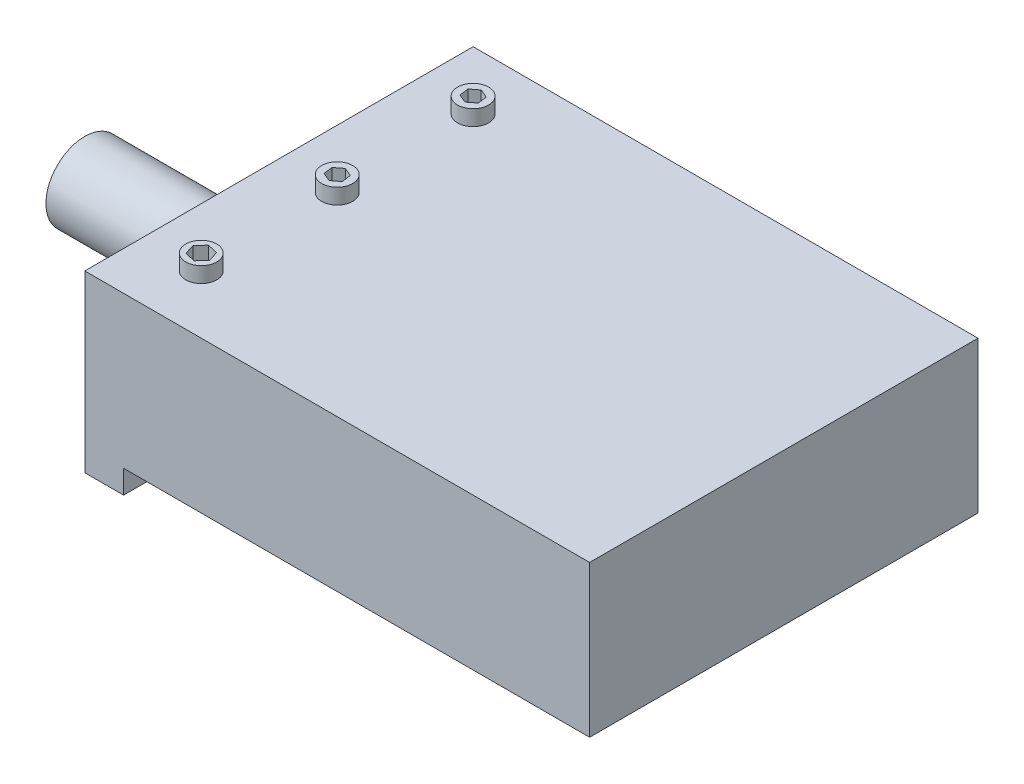
from build123d import *

# Parameters (mm, degrees)
SKETCH1_W           = 70
SKETCH1_H           = 100
BOSS_EXTRUDE1_DEPTH = 30
SKETCH2_R           = 4
BOSS_EXTRUDE2_DEPTH = 4
SKETCH3_R           = 10
BOSS_EXTRUDE3_DEPTH = 50
SKETCH4_W           = 70
SKETCH4_H           = 100
BOSS_EXTRUDE4_DEPTH = 15
SKETCH5_W           = 134.250739562
SKETCH5_H           = 64.864054132
CUT_EXTRUDE1_DEPTH  = 130
CUT_EXTRUDE2_REACH  = 189.566
SKETCH6_W           = 60
SKETCH6_H           = 6
SKETCH7_W           = 100
SKETCH7_H           = 39
BOSS_EXTRUDE5_DEPTH = 60


with BuildPart() as part:
    # Sketch1 → Boss-Extrude1 (new body)
    with BuildSketch(Plane(origin=(0, 0, 0), x_dir=(1, 0, 0), z_dir=(0, 1, 0))):
        Rectangle(SKETCH1_W, SKETCH1_H)
    extrude(amount=BOSS_EXTRUDE1_DEPTH)

    # Sketch2 → Boss-Extrude2 (add)
    # profile 1 of 3: a face of its own
    with BuildSketch(Plane(origin=(0, 30, 0), x_dir=(1, 0, 0), z_dir=(0, 1, 0))):
        with Locations(Location((20, -35, 0), (0, 0, 270))):
            Circle(SKETCH2_R)
        Polygon((21.913058762, -37.035169602), (22.719037957, -34.360827314), (20.805979195, -32.325657712), (18.086941238, -32.964830398), (17.280962043, -35.639172686), (19.194020805, -37.674342288), align=None, mode=Mode.SUBTRACT)
    # profile 2 of 3: a face of its own
    with BuildSketch(Plane(origin=(0, 30, 0), x_dir=(1, 0, 0), z_dir=(0, 1, 0))):
        with Locations(Location((20, 0, 0), (0, 0, 270))):
            Circle(SKETCH2_R)
        Polygon((21.913058762, -1.47020522), (22.229764451, 0.921654877), (20.316705689, 2.391860097), (18.086941238, 1.47020522), (17.770235549, -0.921654877), (19.683294311, -2.391860097), align=None, mode=Mode.SUBTRACT)
    # profile 3 of 3: a face of its own
    with BuildSketch(Plane(origin=(0, 30, 0), x_dir=(1, 0, 0), z_dir=(0, 1, 0))):
        with Locations(Location((20, 35, 0), (0, 0, 270))):
            Circle(SKETCH2_R)
        Polygon((21.913058762, 33.534680981), (22.225532876, 35.924097978), (20.312474114, 37.389416996), (18.086941238, 36.465319019), (17.774467124, 34.075902022), (19.687525886, 32.610583004), align=None, mode=Mode.SUBTRACT)
    extrude(amount=BOSS_EXTRUDE2_DEPTH)

    # Sketch3 → Boss-Extrude3 (add)
    with BuildSketch(Plane(origin=(35, 0, 0), x_dir=(0, 0, -1), z_dir=(1, 0, 0))):
        Circle(SKETCH3_R)
    extrude(amount=BOSS_EXTRUDE3_DEPTH)

    # Sketch4 → Boss-Extrude4 (add)
    with BuildSketch(Plane.XZ):
        Rectangle(SKETCH4_W, SKETCH4_H)
    extrude(amount=BOSS_EXTRUDE4_DEPTH)

    # Mirror1: part across plane


with BuildPart() as part_1:
    add(part.part)
    add(part.part.mirror(Plane(origin=(-35, 30, -50), x_dir=(0, 0, 1), z_dir=(1, 0, 0))))

    # Sketch5 → Cut-Extrude1 (cut)
    with BuildSketch(Plane.ZY.offset(35)):
        with Locations((0.773607985, 10.636315649)):
            Rectangle(SKETCH5_W, SKETCH5_H)
    extrude(amount=-CUT_EXTRUDE1_DEPTH, mode=Mode.SUBTRACT)

    # Sketch6 → Cut-Extrude2 (cut, up to next)
    with BuildSketch(Plane.XY.offset(50), mode=Mode.PRIVATE) as cut_extrude2_sk1:
        with Locations((-65, -12)):
            Rectangle(SKETCH6_W, SKETCH6_H)
    cut_extrude2_tool1 = extrude(cut_extrude2_sk1.sketch, amount=-CUT_EXTRUDE2_REACH, mode=Mode.PRIVATE) & part_1.part
    add(cut_extrude2_tool1.solids().sort_by_distance((-65, -12, 50))[0], mode=Mode.SUBTRACT)

    # Sketch7 → Boss-Extrude5 (add)
    with BuildSketch(Plane(origin=(-35, 0, 0), x_dir=(0, 0, -1), z_dir=(1, 0, 0))):
        with Locations((0, 10.5)):
            Rectangle(SKETCH7_W, SKETCH7_H)
    extrude(amount=BOSS_EXTRUDE5_DEPTH)


solid = part_1.part
